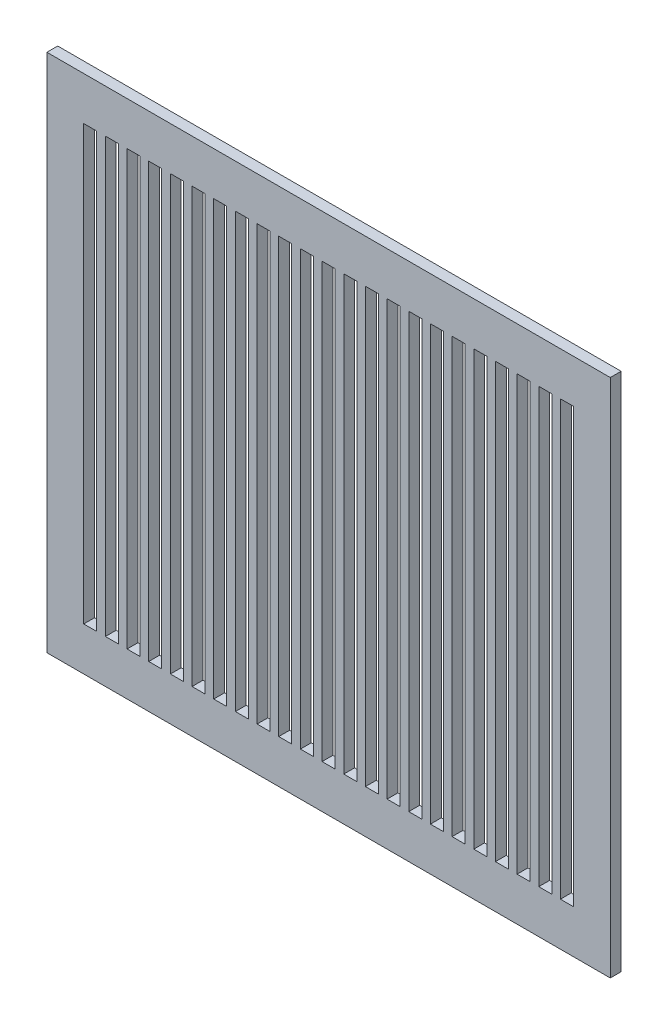
SolidWorks part; units mm, degrees
ref_plane "前视基准面" through (0, 0, 0) normal (0, 0, 1) x (1, 0, 0)
ref_plane "上视基准面" through (0, 0, 0) normal (0, 1, 0) x (1, 0, 0)
ref_plane "右视基准面" through (0, 0, 0) normal (1, 0, 0) x (0, 0, -1)
sketch "草图1" plane through (0, 0, 0) normal (0, 0, 1) x (1, 0, 0)
  line L1 (-130, -120) -> (130, -120)
  line L2 (-130, -120) -> (-130, 120)
  line L3 (-130, 120) -> (130, 120)
  line L4 (130, -120) -> (130, 120)
  line L5 (-130, -120) -> (130, 120) construction
  line L6 (-130, 120) -> (130, -120) construction
  point P0 (0, 0)
  dimension "D1" = 260
  dimension "D2" = 240
extrude "凸台-拉伸1" add sketch "草图1" along normal blind 5
sketch "草图2" plane through (0, 0, 5) normal (0, 0, 1) x (1, 0, 0)
  line L1 (-3, -100) -> (3, -100)
  line L2 (-3, -100) -> (-3, 100)
  line L3 (-3, 100) -> (3, 100)
  line L4 (3, -100) -> (3, 100)
  line L5 (-3, -100) -> (3, 100) construction
  line L6 (-3, 100) -> (3, -100) construction
  point P0 (0, 0)
  dimension "D1" = 6
  dimension "D2" = 200
extrude "切除-拉伸1" cut sketch "草图2" against normal through all
pattern_linear "阵列(线性)1" count 12 spacing 10 along (1, 0, 0) count 12 spacing 10 along (-1, 0, 0) of "切除-拉伸1"
